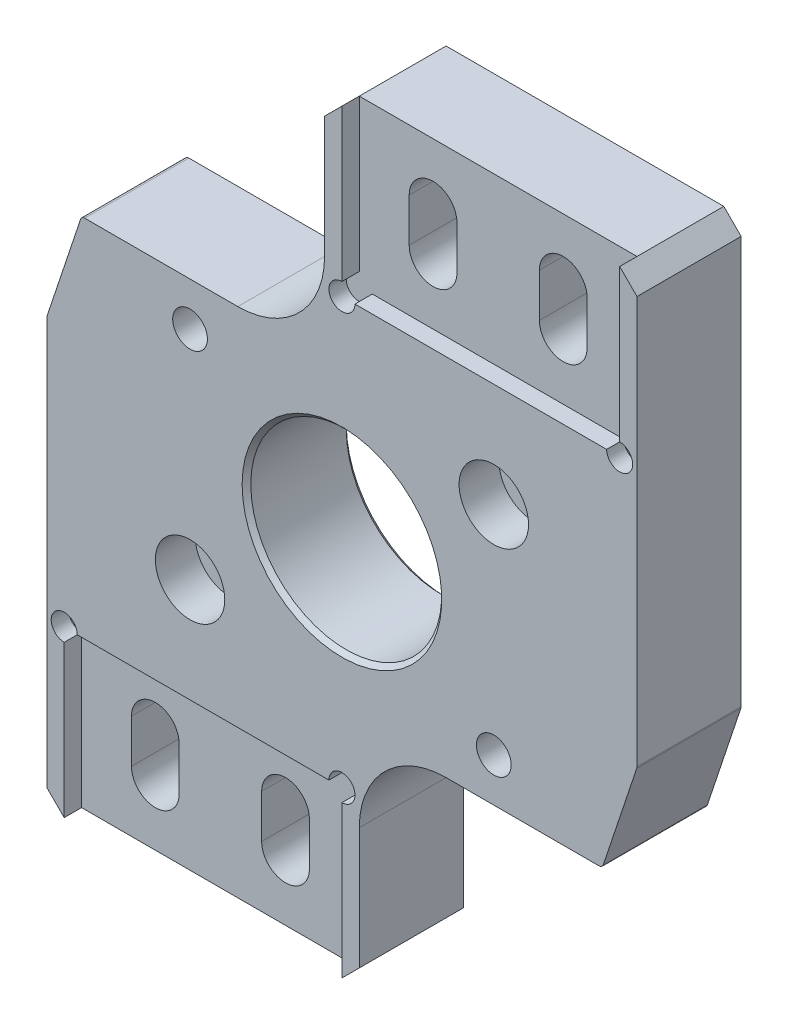
SolidWorks part; units mm, degrees
material "A7075-T6"
ref_plane "Front Plane" through (0, 0, 0) normal (0, 0, 1) x (1, 0, 0)
ref_plane "Top Plane" through (0, 0, 0) normal (0, 1, 0) x (1, 0, 0)
ref_plane "Right Plane" through (0, 0, 0) normal (1, 0, 0) x (0, 0, -1)
sketch "Sketch1" plane through (0, 0, 0) normal (0, 0, 1) x (1, 0, 0)
  line L1 (-34, -43.5) -> (34, -43.5)
  line L2 (-34, -43.5) -> (-34, 43.5)
  line L3 (-34, 43.5) -> (34, 43.5)
  line L4 (34, -43.5) -> (34, 43.5)
  line L5 (-34, -43.5) -> (34, 43.5) construction
  line L6 (-34, 43.5) -> (34, -43.5) construction
  point P0 (0, 0)
  dimension "D1" = 87
  dimension "D2" = 68
extrude "Boss-Extrude1" add sketch "Sketch1" along normal blind 12
sketch "Sketch3" plane through (0, 0, 12) normal (0, 0, 1) x (1, 0, 0)
  line L1 (-2, 43.5) -> (-34, 43.5)
  line L2 (-2, 43.5) -> (-2, 17.5)
  line L3 (-2, 17.5) -> (-34, 17.5)
  line L4 (-34, 43.5) -> (-34, 17.5)
  line L5 (2, -43.5) -> (34, -43.5)
  line L6 (2, -43.5) -> (2, -17.5)
  line L7 (2, -17.5) -> (34, -17.5)
  line L8 (34, -43.5) -> (34, -17.5)
  circle A0 centre (0, 0) radius 11
  dimension "D3" = 22
  dimension "D1" = 26
  dimension "D2" = 32
extrude "Cut-Extrude2" cut sketch "Sketch3" against normal through all
sketch "Sketch16" plane through (0, 0, 12) normal (0, 0, 1) x (1, 0, 0)
  line L0 (-34, -43.5) -> (2, -43.5) construction
  line L1 (0, -43.5) -> (-32, -43.5)
  line L2 (0, -43.5) -> (0, -26)
  line L3 (-1.5, -24.5) -> (-30.5, -24.5)
  line L4 (-32, -43.5) -> (-32, -26)
  line L5 (34, 43.5) -> (-2, 43.5) construction
  line L6 (32, 43.5) -> (0, 43.5)
  line L7 (32, 43.5) -> (32, 26)
  line L8 (30.5, 24.5) -> (1.5, 24.5)
  line L9 (0, 43.5) -> (0, 26)
  line L10 (-16, -43.5) -> (-16, 1.9305) construction
  line L11 (16, 43.5) -> (16, 12.0705) construction
  arc A0 (-30.5, -24.5) -> (-32, -26) centre (-32, -24.5) ccw
  arc A1 (0, -26) -> (-1.5, -24.5) centre (0, -24.5) ccw
  arc A2 (0, 26) -> (1.5, 24.5) centre (0, 24.5) ccw
  arc A3 (30.5, 24.5) -> (32, 26) centre (32, 24.5) ccw
  dimension "D3" = 3
  dimension "D1" = 32
  dimension "D2" = 19
extrude "Cut-Extrude5" cut sketch "Sketch16" against normal blind 2
fillet "Fillet1" radius 10 2 edges at (2, -17.5, 6) (-2, 17.5, 6)
chamfer "Chamfer1" distance 2 angle 45 4 edges at (-34, -43.5, 6) (2, -43.5, 6) (34, 43.5, 6) (-2, 43.5, 6)
sketch "Sketch17" plane through (0, 0, 0) normal (0, 0, -1) x (-1, 0, 0)
  line L0 (-23.5, 36.5) -> (-23.5, 31.5) construction
  line L1 (-20.75, 36.5) -> (-20.75, 31.5)
  line L2 (-26.25, 36.5) -> (-26.25, 31.5)
  line L3 (-8.5, 36.5) -> (-8.5, 31.5) construction
  line L4 (-5.75, 36.5) -> (-5.75, 31.5)
  line L5 (-11.25, 36.5) -> (-11.25, 31.5)
  line L6 (23.5, -31.5) -> (23.5, -36.5) construction
  line L7 (26.25, -31.5) -> (26.25, -36.5)
  line L8 (20.75, -31.5) -> (20.75, -36.5)
  line L9 (8.5, -31.5) -> (8.5, -36.5) construction
  line L10 (11.25, -31.5) -> (11.25, -36.5)
  line L11 (5.75, -31.5) -> (5.75, -36.5)
  line L12 (-16, 43.5) -> (-16, 23.8205) construction
  line L13 (-32, 43.5) -> (0, 43.5) construction
  line L14 (16, -43.5) -> (16, -18.5461) construction
  line L15 (32, -43.5) -> (0, -43.5) construction
  arc A0 (-20.75, 36.5) -> (-26.25, 36.5) centre (-23.5, 36.5) ccw
  arc A1 (-26.25, 31.5) -> (-20.75, 31.5) centre (-23.5, 31.5) ccw
  arc A2 (-5.75, 36.5) -> (-11.25, 36.5) centre (-8.5, 36.5) ccw
  arc A3 (-11.25, 31.5) -> (-5.75, 31.5) centre (-8.5, 31.5) ccw
  arc A4 (26.25, -31.5) -> (20.75, -31.5) centre (23.5, -31.5) ccw
  arc A5 (20.75, -36.5) -> (26.25, -36.5) centre (23.5, -36.5) ccw
  arc A6 (11.25, -31.5) -> (5.75, -31.5) centre (8.5, -31.5) ccw
  arc A7 (5.75, -36.5) -> (11.25, -36.5) centre (8.5, -36.5) ccw
  point P2 (-23.5, 34)
  point P7 (-8.5, 34)
  point P14 (23.5, -34)
  point P21 (8.5, -34)
  dimension "D1" = 2.75
  dimension "D2" = 15
  dimension "D6" = 7
  dimension "D3" = 7
  dimension "D4" = 5
  dimension "D5" = 15
extrude "Cut-Extrude6" cut sketch "Sketch17" against normal through all
chamfer "Chamfer2" distance 12 distance2 4 2 edges at (34, -17.5, 6) (-34, 17.5, 6)
fillet "Fillet3" radius 0.5 4 edges at (-34, 5.5, 6) (-30, 17.5, 6) (30, -17.5, 6) (34, -5.5, 6)
hole_wizard "Hole size by socket head cap screw type1" positions "Sketch13" profile "Sketch12" counterbore size "M4" standard "Gb" end condition through all
sketch "Sketch13" plane through (0, 0, 12) normal (0, 0, 1) x (1, 0, 0)
  line L1 (-17.5, -12.5) -> (17.5, -12.5) construction
  line L2 (-17.5, -12.5) -> (-17.5, 12.5) construction
  line L3 (-17.5, 12.5) -> (17.5, 12.5) construction
  line L4 (17.5, -12.5) -> (17.5, 12.5) construction
  line L5 (-17.5, -12.5) -> (17.5, 12.5) construction
  line L6 (-17.5, 12.5) -> (17.5, -12.5) construction
  point P0 (17.5, 12.5)
  point P4 (-17.5, -12.5)
  dimension "D1" = 35
  dimension "D2" = 25
sketch "Sketch12" plane through (17.5, 12.5, 12) normal (1, 0, 0) x (0, -1, 0)
  line L0 (0, 0) -> (0, 12)
  line L1 (0, 12) -> (2.25, 12)
  line L3 (2.25, 12) -> (2.25, 4.6)
  line L4 (2.25, 4.6) -> (4, 4.6)
  line L5 (4, 4.6) -> (4, 0)
  line L7 (4, 0) -> (0, 0)
  line L11 (0, -6.35) -> (0, 107.95) construction
  dimension "通孔孔直径" = 4.5
  dimension "通孔孔深度" = 12
  dimension "柱形沉头孔直径" = 8
  dimension "柱形沉头孔深度" = 4.6
sketch "Sketch15" plane through (0, 0, 12) normal (0, 0, 1) x (1, 0, 0)
  line L1 (-17.5, -12.5) -> (17.5, -12.5) construction
  line L2 (-17.5, -12.5) -> (-17.5, 12.5) construction
  line L3 (-17.5, 12.5) -> (17.5, 12.5) construction
  line L4 (17.5, -12.5) -> (17.5, 12.5) construction
  line L5 (-17.5, -12.5) -> (17.5, 12.5) construction
  line L6 (-17.5, 12.5) -> (17.5, -12.5) construction
  circle A0 centre (17.5, -12.5) radius 2
  circle A1 centre (-17.5, 12.5) radius 2
  point P2 (0, 0)
  dimension "D1" = 4
extrude "Cut-Extrude4" cut sketch "Sketch15" against normal blind 25
chamfer "Chamfer3" distance 0.5 angle 45 2 edges at (11, 0, 0) (11, 0, 12)
